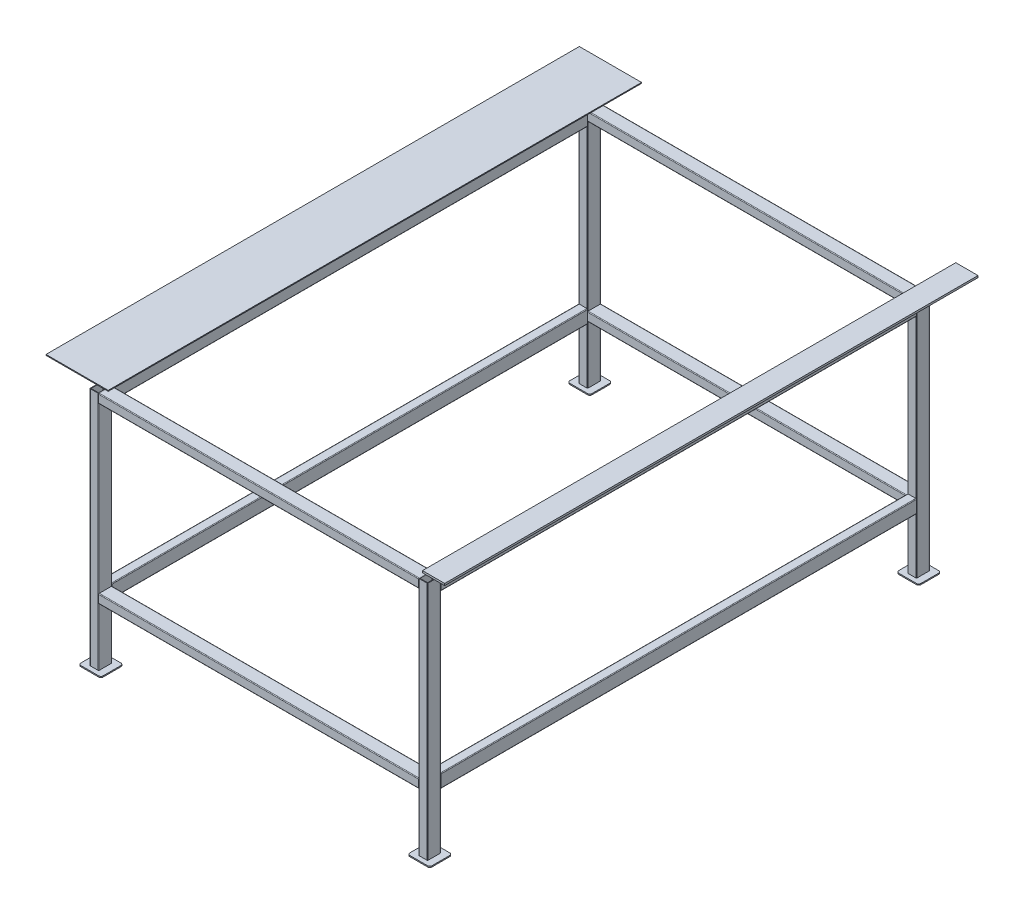
from build123d import *

# Parameters (mm, degrees)
EXTRUDE_1_DEPTH          = 1080
EXTRUDE_1_2_DEPTH        = 1080
EXTRUDE_1_3_DEPTH        = 1080
EXTRUDE_1_4_DEPTH        = 1080
EXTRUDE_2_DEPTH          = 5
EXTRUDE_2_2_DEPTH        = 5
EXTRUDE_2_3_DEPTH        = 5
EXTRUDE_2_4_DEPTH        = 5
EXTRUDE_3_DEPTH          = 2140
EXTRUDE_4_DEPTH          = 1440
EXTRUDE_4_2_DEPTH        = 1440
EXTRUDE_4_3_DEPTH        = 1440
EXTRUDE_4_4_DEPTH        = 1440
EXTRUDE_5_DEPTH          = 2140
EXTRUDE_5_2_DEPTH        = 2140
SKETCH_6_W               = 100
SKETCH_6_H               = 2600
EXTRUDE_6_DEPTH          = 4
EXTRUDE_6_2_DEPTH        = 4
SKETCH_8_W               = 100
SKETCH_8_H               = 2600
EXTRUDE_8_DEPTH          = 4.5
SKETCH_9_W               = 180
SKETCH_9_H               = 2600
EXTRUDE_9_DEPTH          = 4
CUT_EXTRUDE_1_DEPTH      = 142
CUT_EXTRUDE_1_DEPTH_BACK = 4
SKETCH_10_W              = 1794
SKETCH_10_H              = 200


with BuildPart() as part:
    # 草图1 → 凸台-拉伸1 (new body)
    with BuildSketch(Plane(origin=(0, 0, 0), x_dir=(1, 0, 0), z_dir=(0, 1, 0))):
        with BuildLine():
            Line((723, 1130), (757, 1130))
            ThreePointArc((757, 1130), (759.121320344, 1129.121320344), (760, 1127))
            Line((760, 1127), (760, 1073))
            ThreePointArc((760, 1073), (759.121320344, 1070.878679656), (757, 1070))
            Line((757, 1070), (723, 1070))
            ThreePointArc((723, 1070), (720.878679656, 1070.878679656), (720, 1073))
            Line((720, 1073), (720, 1127))
            ThreePointArc((720, 1127), (720.878679656, 1129.121320344), (723, 1130))
        make_face()
        with BuildLine():
            Line((723, 1127.1), (757, 1127.1))
            ThreePointArc((757, 1127.1), (757.070710678, 1127.070710678), (757.1, 1127))
            Line((757.1, 1127), (757.1, 1073))
            ThreePointArc((757.1, 1073), (757.070710678, 1072.929289322), (757, 1072.9))
            Line((757, 1072.9), (723, 1072.9))
            ThreePointArc((723, 1072.9), (722.929289322, 1072.929289322), (722.9, 1073))
            Line((722.9, 1073), (722.9, 1127))
            ThreePointArc((722.9, 1127), (722.929289322, 1127.070710678), (723, 1127.1))
        make_face(mode=Mode.SUBTRACT)
    extrude(amount=EXTRUDE_1_DEPTH)



with BuildPart() as body_2:
    # 草图1 → Extrude 1 2 (new body)
    with BuildSketch(Plane(origin=(0, 0, 0), x_dir=(1, 0, 0), z_dir=(0, 1, 0))):
        with BuildLine():
            Line((723, -1070), (757, -1070))
            ThreePointArc((757, -1070), (759.121320344, -1070.878679656), (760, -1073))
            Line((760, -1073), (760, -1127))
            ThreePointArc((760, -1127), (759.121320344, -1129.121320344), (757, -1130))
            Line((757, -1130), (723, -1130))
            ThreePointArc((723, -1130), (720.878679656, -1129.121320344), (720, -1127))
            Line((720, -1127), (720, -1073))
            ThreePointArc((720, -1073), (720.878679656, -1070.878679656), (723, -1070))
        make_face()
        with BuildLine():
            Line((723, -1072.9), (757, -1072.9))
            ThreePointArc((757, -1072.9), (757.070710678, -1072.929289322), (757.1, -1073))
            Line((757.1, -1073), (757.1, -1127))
            ThreePointArc((757.1, -1127), (757.070710678, -1127.070710678), (757, -1127.1))
            Line((757, -1127.1), (723, -1127.1))
            ThreePointArc((723, -1127.1), (722.929289322, -1127.070710678), (722.9, -1127))
            Line((722.9, -1127), (722.9, -1073))
            ThreePointArc((722.9, -1073), (722.929289322, -1072.929289322), (723, -1072.9))
        make_face(mode=Mode.SUBTRACT)
    extrude(amount=EXTRUDE_1_2_DEPTH)


with BuildPart() as body_3:
    # 草图1 → Extrude 1 3 (new body)
    with BuildSketch(Plane(origin=(0, 0, 0), x_dir=(1, 0, 0), z_dir=(0, 1, 0))):
        with BuildLine():
            Line((-757, -1070), (-723, -1070))
            ThreePointArc((-723, -1070), (-720.878679656, -1070.878679656), (-720, -1073))
            Line((-720, -1073), (-720, -1127))
            ThreePointArc((-720, -1127), (-720.878679656, -1129.121320344), (-723, -1130))
            Line((-723, -1130), (-757, -1130))
            ThreePointArc((-757, -1130), (-759.121320344, -1129.121320344), (-760, -1127))
            Line((-760, -1127), (-760, -1073))
            ThreePointArc((-760, -1073), (-759.121320344, -1070.878679656), (-757, -1070))
        make_face()
        with BuildLine():
            Line((-757, -1072.9), (-723, -1072.9))
            ThreePointArc((-723, -1072.9), (-722.929289322, -1072.929289322), (-722.9, -1073))
            Line((-722.9, -1073), (-722.9, -1127))
            ThreePointArc((-722.9, -1127), (-722.929289322, -1127.070710678), (-723, -1127.1))
            Line((-723, -1127.1), (-757, -1127.1))
            ThreePointArc((-757, -1127.1), (-757.070710678, -1127.070710678), (-757.1, -1127))
            Line((-757.1, -1127), (-757.1, -1073))
            ThreePointArc((-757.1, -1073), (-757.070710678, -1072.929289322), (-757, -1072.9))
        make_face(mode=Mode.SUBTRACT)
    extrude(amount=EXTRUDE_1_3_DEPTH)


with BuildPart() as body_4:
    # 草图1 → Extrude 1 4 (new body)
    with BuildSketch(Plane(origin=(0, 0, 0), x_dir=(1, 0, 0), z_dir=(0, 1, 0))):
        with BuildLine():
            Line((-757, 1130), (-723, 1130))
            ThreePointArc((-723, 1130), (-720.878679656, 1129.121320344), (-720, 1127))
            Line((-720, 1127), (-720, 1073))
            ThreePointArc((-720, 1073), (-720.878679656, 1070.878679656), (-723, 1070))
            Line((-723, 1070), (-757, 1070))
            ThreePointArc((-757, 1070), (-759.121320344, 1070.878679656), (-760, 1073))
            Line((-760, 1073), (-760, 1127))
            ThreePointArc((-760, 1127), (-759.121320344, 1129.121320344), (-757, 1130))
        make_face()
        with BuildLine():
            Line((-757, 1127.1), (-723, 1127.1))
            ThreePointArc((-723, 1127.1), (-722.929289322, 1127.070710678), (-722.9, 1127))
            Line((-722.9, 1127), (-722.9, 1073))
            ThreePointArc((-722.9, 1073), (-722.929289322, 1072.929289322), (-723, 1072.9))
            Line((-723, 1072.9), (-757, 1072.9))
            ThreePointArc((-757, 1072.9), (-757.070710678, 1072.929289322), (-757.1, 1073))
            Line((-757.1, 1073), (-757.1, 1127))
            ThreePointArc((-757.1, 1127), (-757.070710678, 1127.070710678), (-757, 1127.1))
        make_face(mode=Mode.SUBTRACT)
    extrude(amount=EXTRUDE_1_4_DEPTH)


with BuildPart() as body_5:
    # 草图2 → 凸台-拉伸2 (new body)
    with BuildSketch(Plane.XZ):
        with BuildLine():
            Line((-780, -1050), (-700, -1050))
            ThreePointArc((-700, -1050), (-692.928932188, -1052.928932188), (-690, -1060))
            Line((-690, -1060), (-690, -1140))
            ThreePointArc((-690, -1140), (-692.928932188, -1147.071067812), (-700, -1150))
            Line((-700, -1150), (-780, -1150))
            ThreePointArc((-780, -1150), (-787.071067812, -1147.071067812), (-790, -1140))
            Line((-790, -1140), (-790, -1060))
            ThreePointArc((-790, -1060), (-787.071067812, -1052.928932188), (-780, -1050))
        make_face()
    extrude(amount=EXTRUDE_2_DEPTH)


with BuildPart() as body_6:
    # 草图2 → Extrude 2 2 (new body)
    with BuildSketch(Plane.XZ):
        with BuildLine():
            Line((-690, 1060), (-690, 1140))
            ThreePointArc((-690, 1140), (-692.928932188, 1147.071067812), (-700, 1150))
            Line((-700, 1150), (-780, 1150))
            ThreePointArc((-780, 1150), (-787.071067812, 1147.071067812), (-790, 1140))
            Line((-790, 1140), (-790, 1060))
            ThreePointArc((-790, 1060), (-787.071067812, 1052.928932188), (-780, 1050))
            Line((-780, 1050), (-700, 1050))
            ThreePointArc((-700, 1050), (-692.928932188, 1052.928932188), (-690, 1060))
        make_face()
    extrude(amount=EXTRUDE_2_2_DEPTH)


with BuildPart() as body_7:
    # 草图2 → Extrude 2 3 (new body)
    with BuildSketch(Plane.XZ):
        with BuildLine():
            Line((780, 1050), (700, 1050))
            ThreePointArc((700, 1050), (692.928932188, 1052.928932188), (690, 1060))
            Line((690, 1060), (690, 1140))
            ThreePointArc((690, 1140), (692.928932188, 1147.071067812), (700, 1150))
            Line((700, 1150), (780, 1150))
            ThreePointArc((780, 1150), (787.071067812, 1147.071067812), (790, 1140))
            Line((790, 1140), (790, 1060))
            ThreePointArc((790, 1060), (787.071067812, 1052.928932188), (780, 1050))
        make_face()
    extrude(amount=EXTRUDE_2_3_DEPTH)


with BuildPart() as body_8:
    # 草图2 → Extrude 2 4 (new body)
    with BuildSketch(Plane.XZ):
        with BuildLine():
            Line((690, -1060), (690, -1140))
            ThreePointArc((690, -1140), (692.928932188, -1147.071067812), (700, -1150))
            Line((700, -1150), (780, -1150))
            ThreePointArc((780, -1150), (787.071067812, -1147.071067812), (790, -1140))
            Line((790, -1140), (790, -1060))
            ThreePointArc((790, -1060), (787.071067812, -1052.928932188), (780, -1050))
            Line((780, -1050), (700, -1050))
            ThreePointArc((700, -1050), (692.928932188, -1052.928932188), (690, -1060))
        make_face()
    extrude(amount=EXTRUDE_2_4_DEPTH)


with BuildPart() as part_1:
    add(part.part)

    add(body_2.part)  # 凸台-拉伸3 merges body 2

    add(body_3.part)  # 凸台-拉伸3 merges body 3

    add(body_4.part)  # 凸台-拉伸3 merges body 4
    # 草图3 → 凸台-拉伸3 (add)
    # profile 1 of 2: a face of its own
    with BuildSketch(Plane(origin=(0, 0, 1070), x_dir=(-1, 0, 0), z_dir=(0, 0, -1))):
        with BuildLine():
            Line((-757, 1080), (-723, 1080))
            ThreePointArc((-723, 1080), (-720.878679656, 1079.121320344), (-720, 1077))
            Line((-720, 1077), (-720, 1023))
            ThreePointArc((-720, 1023), (-720.878679656, 1020.878679656), (-723, 1020))
            Line((-723, 1020), (-757, 1020))
            ThreePointArc((-757, 1020), (-759.121320344, 1020.878679656), (-760, 1023))
            Line((-760, 1023), (-760, 1077))
            ThreePointArc((-760, 1077), (-759.121320344, 1079.121320344), (-757, 1080))
        make_face()
        with BuildLine():
            Line((-757, 1077.1), (-723, 1077.1))
            ThreePointArc((-723, 1077.1), (-722.929289322, 1077.070710678), (-722.9, 1077))
            Line((-722.9, 1077), (-722.9, 1023))
            ThreePointArc((-722.9, 1023), (-722.929289322, 1022.929289322), (-723, 1022.9))
            Line((-723, 1022.9), (-757, 1022.9))
            ThreePointArc((-757, 1022.9), (-757.070710678, 1022.929289322), (-757.1, 1023))
            Line((-757.1, 1023), (-757.1, 1077))
            ThreePointArc((-757.1, 1077), (-757.070710678, 1077.070710678), (-757, 1077.1))
        make_face(mode=Mode.SUBTRACT)
    # profile 2 of 2: a face of its own
    with BuildSketch(Plane(origin=(0, 0, 1070), x_dir=(-1, 0, 0), z_dir=(0, 0, -1))):
        with BuildLine():
            Line((723, 1080), (757, 1080))
            ThreePointArc((757, 1080), (759.121320344, 1079.121320344), (760, 1077))
            Line((760, 1077), (760, 1023))
            ThreePointArc((760, 1023), (759.121320344, 1020.878679656), (757, 1020))
            Line((757, 1020), (723, 1020))
            ThreePointArc((723, 1020), (720.878679656, 1020.878679656), (720, 1023))
            Line((720, 1023), (720, 1077))
            ThreePointArc((720, 1077), (720.878679656, 1079.121320344), (723, 1080))
        make_face()
        with BuildLine():
            Line((723, 1077.1), (757, 1077.1))
            ThreePointArc((757, 1077.1), (757.070710678, 1077.070710678), (757.1, 1077))
            Line((757.1, 1077), (757.1, 1023))
            ThreePointArc((757.1, 1023), (757.070710678, 1022.929289322), (757, 1022.9))
            Line((757, 1022.9), (723, 1022.9))
            ThreePointArc((723, 1022.9), (722.929289322, 1022.929289322), (722.9, 1023))
            Line((722.9, 1023), (722.9, 1077))
            ThreePointArc((722.9, 1077), (722.929289322, 1077.070710678), (723, 1077.1))
        make_face(mode=Mode.SUBTRACT)
    extrude(amount=EXTRUDE_3_DEPTH)


with BuildPart() as body_6_2:
    # 草图4 → 凸台-拉伸4 (new body)
    with BuildSketch(Plane.ZY.offset(-720)):
        with BuildLine():
            Line((-1130, 263), (-1130, 297))
            ThreePointArc((-1130, 297), (-1129.121320344, 299.121320344), (-1127, 300))
            Line((-1127, 300), (-1073, 300))
            ThreePointArc((-1073, 300), (-1070.878679656, 299.121320344), (-1070, 297))
            Line((-1070, 297), (-1070, 263))
            ThreePointArc((-1070, 263), (-1070.878679656, 260.878679656), (-1073, 260))
            Line((-1073, 260), (-1127, 260))
            ThreePointArc((-1127, 260), (-1129.121320344, 260.878679656), (-1130, 263))
        make_face()
        with BuildLine():
            Line((-1127.1, 263), (-1127.1, 297))
            ThreePointArc((-1127.1, 297), (-1127.070710678, 297.070710678), (-1127, 297.1))
            Line((-1127, 297.1), (-1073, 297.1))
            ThreePointArc((-1073, 297.1), (-1072.929289322, 297.070710678), (-1072.9, 297))
            Line((-1072.9, 297), (-1072.9, 263))
            ThreePointArc((-1072.9, 263), (-1072.929289322, 262.929289322), (-1073, 262.9))
            Line((-1073, 262.9), (-1127, 262.9))
            ThreePointArc((-1127, 262.9), (-1127.070710678, 262.929289322), (-1127.1, 263))
        make_face(mode=Mode.SUBTRACT)
    extrude(amount=EXTRUDE_4_DEPTH)


with BuildPart() as body_7_2:
    # 草图4 → Extrude 4 2 (new body)
    with BuildSketch(Plane.ZY.offset(-720)):
        with BuildLine():
            Line((-1130, 1043), (-1130, 1077))
            ThreePointArc((-1130, 1077), (-1129.121320344, 1079.121320344), (-1127, 1080))
            Line((-1127, 1080), (-1073, 1080))
            ThreePointArc((-1073, 1080), (-1070.878679656, 1079.121320344), (-1070, 1077))
            Line((-1070, 1077), (-1070, 1043))
            ThreePointArc((-1070, 1043), (-1070.878679656, 1040.878679656), (-1073, 1040))
            Line((-1073, 1040), (-1127, 1040))
            ThreePointArc((-1127, 1040), (-1129.121320344, 1040.878679656), (-1130, 1043))
        make_face()
        with BuildLine():
            Line((-1127.1, 1043), (-1127.1, 1077))
            ThreePointArc((-1127.1, 1077), (-1127.070710678, 1077.070710678), (-1127, 1077.1))
            Line((-1127, 1077.1), (-1073, 1077.1))
            ThreePointArc((-1073, 1077.1), (-1072.929289322, 1077.070710678), (-1072.9, 1077))
            Line((-1072.9, 1077), (-1072.9, 1043))
            ThreePointArc((-1072.9, 1043), (-1072.929289322, 1042.929289322), (-1073, 1042.9))
            Line((-1073, 1042.9), (-1127, 1042.9))
            ThreePointArc((-1127, 1042.9), (-1127.070710678, 1042.929289322), (-1127.1, 1043))
        make_face(mode=Mode.SUBTRACT)
    extrude(amount=EXTRUDE_4_2_DEPTH)


with BuildPart() as body_8_2:
    # 草图4 → Extrude 4 3 (new body)
    with BuildSketch(Plane.ZY.offset(-720)):
        with BuildLine():
            Line((1130, 263), (1130, 297))
            ThreePointArc((1130, 297), (1129.121320344, 299.121320344), (1127, 300))
            Line((1127, 300), (1073, 300))
            ThreePointArc((1073, 300), (1070.878679656, 299.121320344), (1070, 297))
            Line((1070, 297), (1070, 263))
            ThreePointArc((1070, 263), (1070.878679656, 260.878679656), (1073, 260))
            Line((1073, 260), (1127, 260))
            ThreePointArc((1127, 260), (1129.121320344, 260.878679656), (1130, 263))
        make_face()
        with BuildLine():
            Line((1127.1, 263), (1127.1, 297))
            ThreePointArc((1127.1, 297), (1127.070710678, 297.070710678), (1127, 297.1))
            Line((1127, 297.1), (1073, 297.1))
            ThreePointArc((1073, 297.1), (1072.929289322, 297.070710678), (1072.9, 297))
            Line((1072.9, 297), (1072.9, 263))
            ThreePointArc((1072.9, 263), (1072.929289322, 262.929289322), (1073, 262.9))
            Line((1073, 262.9), (1127, 262.9))
            ThreePointArc((1127, 262.9), (1127.070710678, 262.929289322), (1127.1, 263))
        make_face(mode=Mode.SUBTRACT)
    extrude(amount=EXTRUDE_4_3_DEPTH)


with BuildPart() as body_9:
    # 草图4 → Extrude 4 4 (new body)
    with BuildSketch(Plane.ZY.offset(-720)):
        with BuildLine():
            Line((1130, 1043), (1130, 1077))
            ThreePointArc((1130, 1077), (1129.121320344, 1079.121320344), (1127, 1080))
            Line((1127, 1080), (1073, 1080))
            ThreePointArc((1073, 1080), (1070.878679656, 1079.121320344), (1070, 1077))
            Line((1070, 1077), (1070, 1043))
            ThreePointArc((1070, 1043), (1070.878679656, 1040.878679656), (1073, 1040))
            Line((1073, 1040), (1127, 1040))
            ThreePointArc((1127, 1040), (1129.121320344, 1040.878679656), (1130, 1043))
        make_face()
        with BuildLine():
            Line((1127.1, 1043), (1127.1, 1077))
            ThreePointArc((1127.1, 1077), (1127.070710678, 1077.070710678), (1127, 1077.1))
            Line((1127, 1077.1), (1073, 1077.1))
            ThreePointArc((1073, 1077.1), (1072.929289322, 1077.070710678), (1072.9, 1077))
            Line((1072.9, 1077), (1072.9, 1043))
            ThreePointArc((1072.9, 1043), (1072.929289322, 1042.929289322), (1073, 1042.9))
            Line((1073, 1042.9), (1127, 1042.9))
            ThreePointArc((1127, 1042.9), (1127.070710678, 1042.929289322), (1127.1, 1043))
        make_face(mode=Mode.SUBTRACT)
    extrude(amount=EXTRUDE_4_4_DEPTH)


with BuildPart() as body_10:
    # 草图5 → 凸台-拉伸5 (new body)
    with BuildSketch(Plane(origin=(0, 0, 1070), x_dir=(-1, 0, 0), z_dir=(0, 0, -1))):
        with BuildLine():
            Line((-757, 310), (-723, 310))
            ThreePointArc((-723, 310), (-720.878679656, 309.121320344), (-720, 307))
            Line((-720, 307), (-720, 253))
            ThreePointArc((-720, 253), (-720.878679656, 250.878679656), (-723, 250))
            Line((-723, 250), (-757, 250))
            ThreePointArc((-757, 250), (-759.121320344, 250.878679656), (-760, 253))
            Line((-760, 253), (-760, 307))
            ThreePointArc((-760, 307), (-759.121320344, 309.121320344), (-757, 310))
        make_face()
        with BuildLine():
            Line((-757, 307.1), (-723, 307.1))
            ThreePointArc((-723, 307.1), (-722.929289322, 307.070710678), (-722.9, 307))
            Line((-722.9, 307), (-722.9, 253))
            ThreePointArc((-722.9, 253), (-722.929289322, 252.929289322), (-723, 252.9))
            Line((-723, 252.9), (-757, 252.9))
            ThreePointArc((-757, 252.9), (-757.070710678, 252.929289322), (-757.1, 253))
            Line((-757.1, 253), (-757.1, 307))
            ThreePointArc((-757.1, 307), (-757.070710678, 307.070710678), (-757, 307.1))
        make_face(mode=Mode.SUBTRACT)
    extrude(amount=EXTRUDE_5_DEPTH)


with BuildPart() as body_11:
    # 草图5 → Extrude 5 2 (new body)
    with BuildSketch(Plane(origin=(0, 0, 1070), x_dir=(-1, 0, 0), z_dir=(0, 0, -1))):
        with BuildLine():
            Line((757, 310), (723, 310))
            ThreePointArc((723, 310), (720.878679656, 309.121320344), (720, 307))
            Line((720, 307), (720, 253))
            ThreePointArc((720, 253), (720.878679656, 250.878679656), (723, 250))
            Line((723, 250), (757, 250))
            ThreePointArc((757, 250), (759.121320344, 250.878679656), (760, 253))
            Line((760, 253), (760, 307))
            ThreePointArc((760, 307), (759.121320344, 309.121320344), (757, 310))
        make_face()
        with BuildLine():
            Line((757, 307.1), (723, 307.1))
            ThreePointArc((723, 307.1), (722.929289322, 307.070710678), (722.9, 307))
            Line((722.9, 307), (722.9, 253))
            ThreePointArc((722.9, 253), (722.929289322, 252.929289322), (723, 252.9))
            Line((723, 252.9), (757, 252.9))
            ThreePointArc((757, 252.9), (757.070710678, 252.929289322), (757.1, 253))
            Line((757.1, 253), (757.1, 307))
            ThreePointArc((757.1, 307), (757.070710678, 307.070710678), (757, 307.1))
        make_face(mode=Mode.SUBTRACT)
    extrude(amount=EXTRUDE_5_2_DEPTH)


with BuildPart() as body_12:
    # 草图6 → 凸台-拉伸6 (new body)
    with BuildSketch(Plane(origin=(0, 1080, 0), x_dir=(1, 0, 0), z_dir=(0, 1, 0))):
        with Locations((-757, 0)):
            Rectangle(SKETCH_6_W, SKETCH_6_H)
    extrude(amount=EXTRUDE_6_DEPTH)

    # 草图9 → 凸台-拉伸9 (add)
    with BuildSketch(Plane(origin=(0, 1084, 0), x_dir=(1, 0, 0), z_dir=(0, 1, 0))):
        with Locations((-897, 0)):
            Rectangle(SKETCH_9_W, SKETCH_9_H)
    extrude(amount=-EXTRUDE_9_DEPTH)


with BuildPart() as body_13:
    # 草图6 → Extrude 6 2 (new body)
    with BuildSketch(Plane(origin=(0, 1080, 0), x_dir=(1, 0, 0), z_dir=(0, 1, 0))):
        with Locations((757, 0)):
            Rectangle(SKETCH_6_W, SKETCH_6_H)
    extrude(amount=EXTRUDE_6_2_DEPTH)

    # 草图8 → 凸台-拉伸8 (add)
    with BuildSketch(Plane(origin=(0, 1084, 0), x_dir=(1, 0, 0), z_dir=(0, 1, 0))):
        with Locations((757, 0)):
            Rectangle(SKETCH_8_W, SKETCH_8_H)
    extrude(amount=EXTRUDE_8_DEPTH)


with BuildPart() as cut_extrude_1_tool:
    # 草图10 → 切除-拉伸1 (new, two sides: drawn at the far end of the back side and taken through both)
    with BuildSketch(Plane(origin=(0, 1084, 0), x_dir=(1, 0, 0), z_dir=(0, 1, 0)).offset(-CUT_EXTRUDE_1_DEPTH_BACK)):
        with Locations((-90, -1200)):
            Rectangle(SKETCH_10_W, SKETCH_10_H)
    extrude(amount=CUT_EXTRUDE_1_DEPTH + CUT_EXTRUDE_1_DEPTH_BACK)


with BuildPart() as body_12_1:
    add(body_12.part)

    # 切除-拉伸1: cut by cut_extrude_1_tool
    add(cut_extrude_1_tool.part, mode=Mode.SUBTRACT)


with BuildPart() as body_13_1:
    add(body_13.part)

    # 切除-拉伸1: cut by cut_extrude_1_tool
    add(cut_extrude_1_tool.part, mode=Mode.SUBTRACT)


solid = Compound([body_5.part, body_6.part, body_7.part, body_8.part, part_1.part, body_6_2.part, body_7_2.part, body_8_2.part, body_9.part, body_10.part, body_11.part, body_12_1.part, body_13_1.part])
